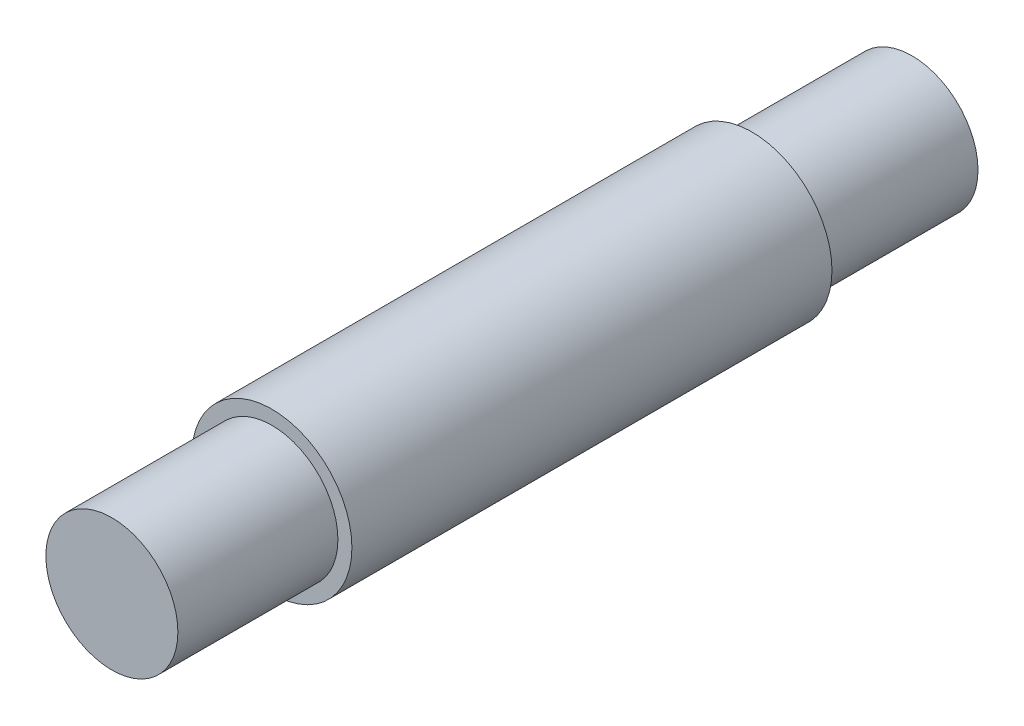
SolidWorks part; units mm, degrees
ref_plane "Front Plane" through (0, 0, 0) normal (0, 0, 1) x (1, 0, 0)
ref_plane "Top Plane" through (0, 0, 0) normal (0, 1, 0) x (1, 0, 0)
ref_plane "Right Plane" through (0, 0, 0) normal (1, 0, 0) x (0, 0, -1)
sketch "Sketch 1" plane through (0, 0, 0) normal (0, 0, 1) x (1, 0, 0)
  line L0 (0, 55.4084) -> (0, -50.1461) construction
  line L1 (-164.9606, 0) -> (173.305, 0) construction
  circle A0 centre (0, 0) radius 20
  dimension "D1" = 40
extrude "Boss-Extrude 1" add sketch "Sketch 1" along normal mid plane 120
sketch "Sketch 2" plane through (0, 0, 60) normal (0, 0, 1) x (1, 0, 0)
  circle A0 centre (0, 0) radius 16.5
  dimension "D1" = 33
extrude "Boss-Extrude 2" add sketch "Sketch 2" along normal blind 40
mirror "Mirror 1" about plane through (0, 0, 0) normal (0, 0, 1) of "Boss-Extrude 2"
